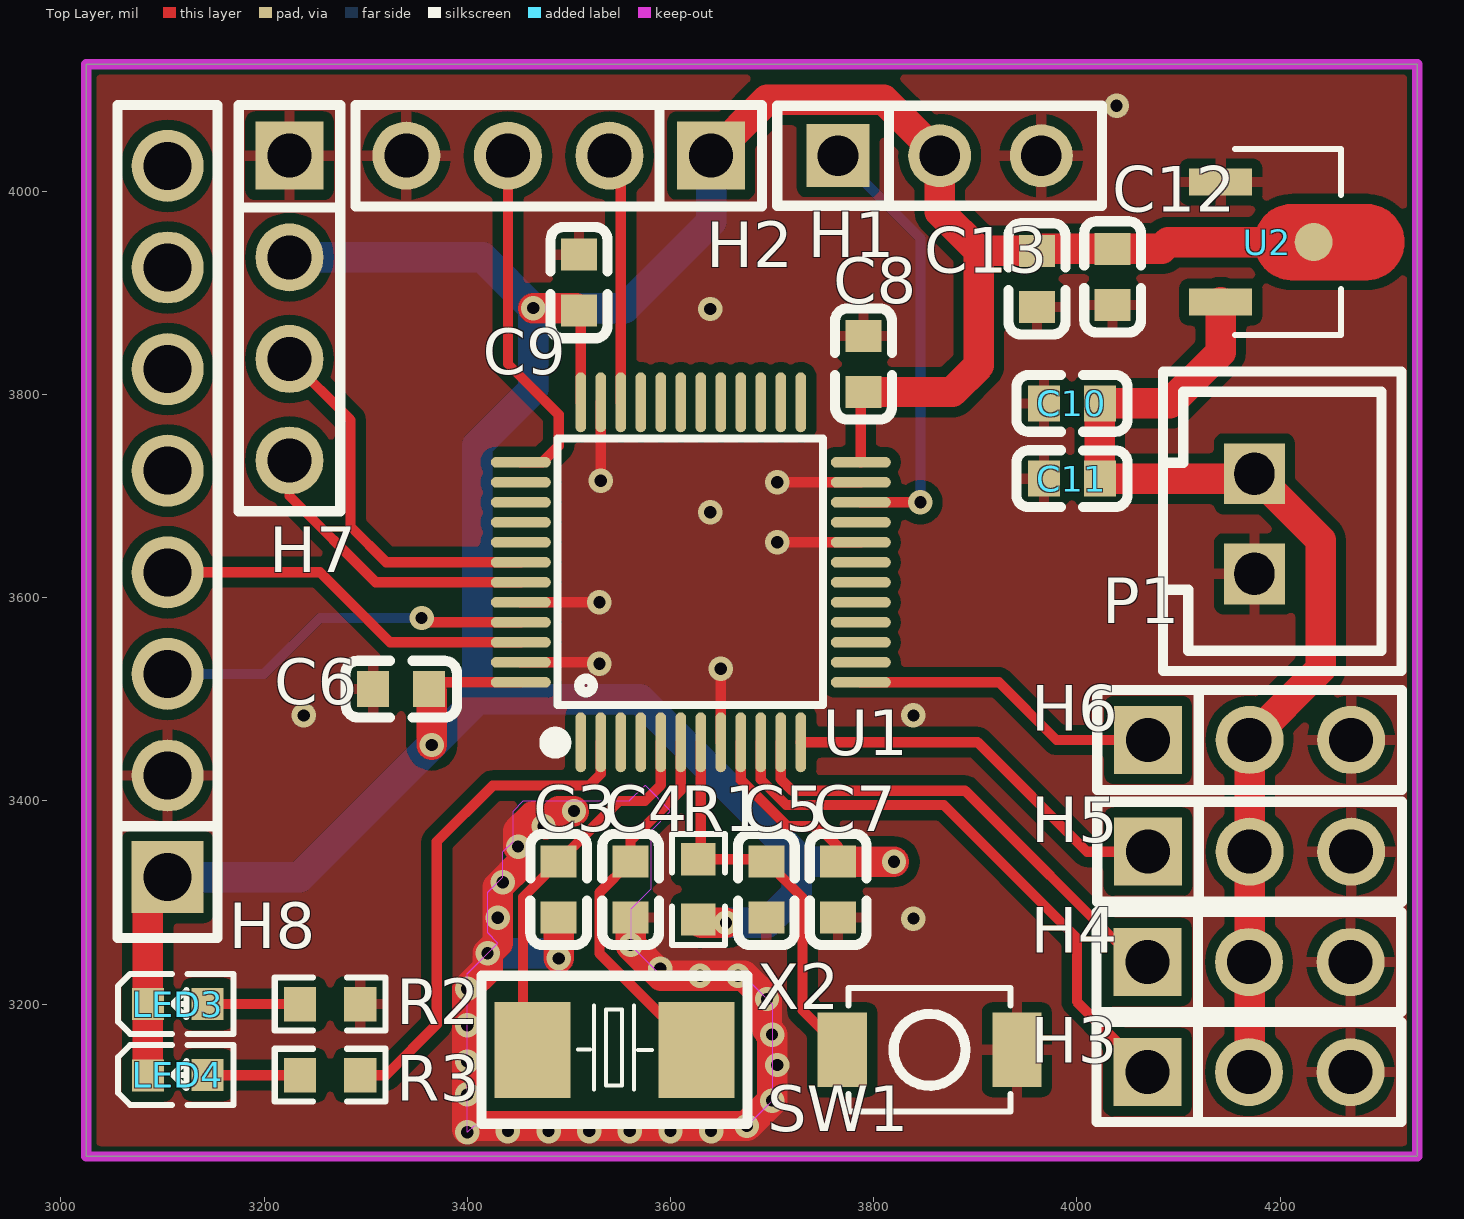
[diagram p0: Top Layer view]
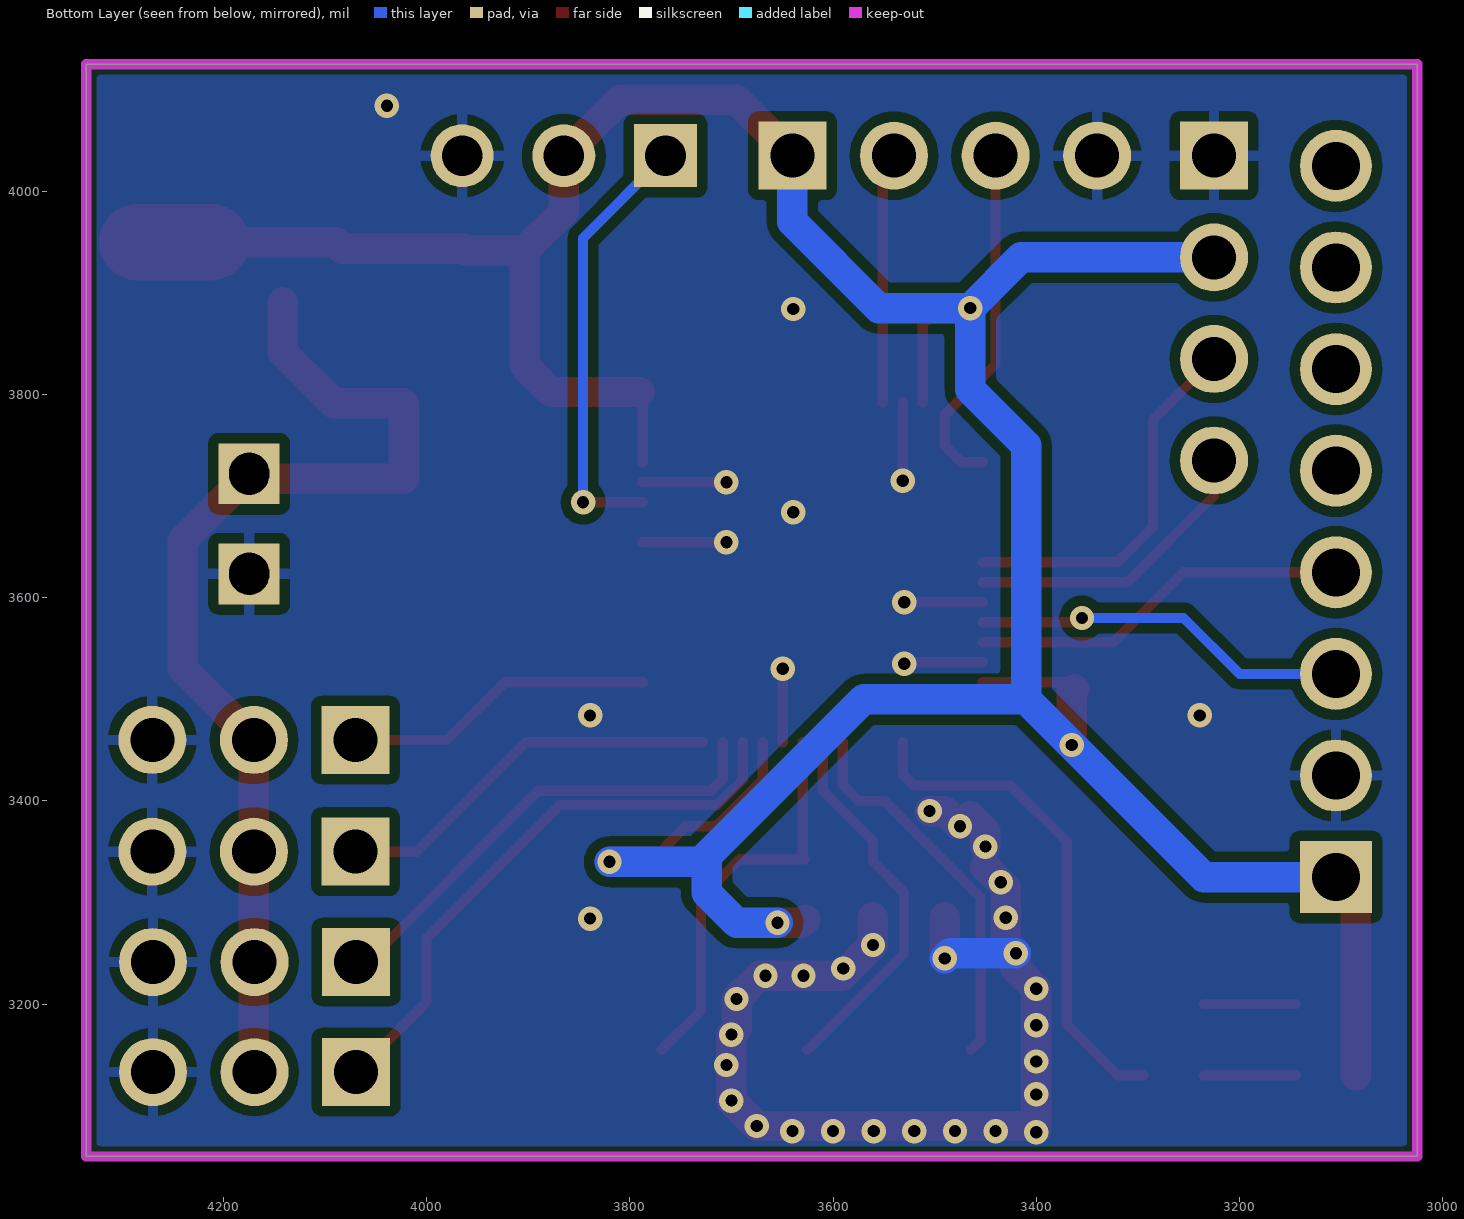
[diagram p1: Bottom Layer view, seen from below]
# Altium PCB MISC51388.pcbdoc
Units mil, origin at the board's own origin, x right, y up, seen from the top; angles counter-clockwise.
Board outline 1310 x 1075 mil, 2 copper layers (Top Layer, Bottom Layer), stack 62.206 mil thick; 29 components, 22 nets, 120 pads, 45 vias.

## Layer stack, top to bottom
Top Solder Mask Layer: solder mask 0.394, Dk 3.3
Top Layer: signal copper 1.379
Dielectric1: surface 59.449, FR4, Dk 4.5
Bottom Layer: signal copper 1.378
Bottom Solder Mask Layer: solder mask 0.394, Dk 3.3

## Board outline
3025,4125 3025,3050 4335,3050 4335,4125

## Design rules (kind name [scope] priority, off if disabled: settings)
BoardOutlineClearance copperThickness2oz_1 [All] p2 off: genericclearance=7.99 ignorepadtopadclearanceinfootprint=FALSE except(0: Arc-SplitContinuation Track-SplitContinuation SMDPad-SplitContinuation THPad-SplitContinuation Via-SplitContinuation Fill-SplitContinuation Region-SplitContinuation Poly-SplitContinuation Text-SplitContinuation Hole-SplitContinuation; 5.98: Arc-CutoutEdge Track-CutoutEdge SMDPad-CutoutEdge THPad-CutoutEdge Via-CutoutEdge Text-CutoutEdge; 6.9: Hole-OutlineEdge Hole-CutoutEdge; 10: Poly-OutlineEdge Poly-CutoutEdge; 11.81: Arc-OutlineEdge Track-OutlineEdge SMDPad-OutlineEdge THPad-OutlineEdge Via-OutlineEdge Fill-OutlineEdge Region-OutlineEdge Text-OutlineEdge Fill-CutoutEdge Region-CutoutEdge)
BoardOutlineClearance Plane_innerPlane_1 [All] p4 off: genericclearance=4.02 ignorepadtopadclearanceinfootprint=FALSE except(0: Arc-SplitContinuation Track-SplitContinuation SMDPad-SplitContinuation THPad-SplitContinuation Via-SplitContinuation Fill-SplitContinuation Region-SplitContinuation Poly-SplitContinuation Text-SplitContinuation Hole-SplitContinuation; 5.98: SMDPad-CutoutEdge THPad-CutoutEdge Via-CutoutEdge Fill-CutoutEdge Region-CutoutEdge Text-CutoutEdge; 6.93: Hole-OutlineEdge Hole-CutoutEdge; 10: Poly-OutlineEdge Poly-CutoutEdge; 11.81: Arc-OutlineEdge Track-OutlineEdge SMDPad-OutlineEdge THPad-OutlineEdge Via-OutlineEdge Fill-OutlineEdge Region-OutlineEdge Text-OutlineEdge Arc-CutoutEdge Track-CutoutEdge)
BoardOutlineClearance Copper_copperRegion_1 [All] p6 off: genericclearance=4.02 ignorepadtopadclearanceinfootprint=FALSE except(0: Arc-SplitContinuation Track-SplitContinuation SMDPad-SplitContinuation THPad-SplitContinuation Via-SplitContinuation Fill-SplitContinuation Region-SplitContinuation Poly-SplitContinuation Text-SplitContinuation Hole-SplitContinuation; 5.98: SMDPad-CutoutEdge THPad-CutoutEdge Via-CutoutEdge Fill-CutoutEdge Region-CutoutEdge Text-CutoutEdge; 6.93: Hole-OutlineEdge Hole-CutoutEdge; 10: Poly-OutlineEdge Poly-CutoutEdge; 11.81: Arc-OutlineEdge Track-OutlineEdge SMDPad-OutlineEdge THPad-OutlineEdge Via-OutlineEdge Fill-OutlineEdge Region-OutlineEdge Text-OutlineEdge Arc-CutoutEdge Track-CutoutEdge)
BoardOutlineClearance copperThickness1oz_1 [All] p8: genericclearance=4.02 ignorepadtopadclearanceinfootprint=FALSE except(0: Arc-SplitContinuation Track-SplitContinuation SMDPad-SplitContinuation THPad-SplitContinuation Via-SplitContinuation Fill-SplitContinuation Region-SplitContinuation Poly-SplitContinuation Text-SplitContinuation Hole-SplitContinuation; 5.98: SMDPad-CutoutEdge THPad-CutoutEdge Via-CutoutEdge Fill-CutoutEdge Region-CutoutEdge Text-CutoutEdge; 6.93: Hole-OutlineEdge Hole-CutoutEdge; 10: Poly-OutlineEdge Poly-CutoutEdge; 11.81: Arc-OutlineEdge Track-OutlineEdge SMDPad-OutlineEdge THPad-OutlineEdge Via-OutlineEdge Fill-OutlineEdge Region-OutlineEdge Text-OutlineEdge Arc-CutoutEdge Track-CutoutEdge)
Clearance copperThickness2oz [All] p1 off: gap=7.99 ignorepadtopadclearanceinfootprint=FALSE except(5.98: SMDPad-Track SMDPad-SMDPad THPad-Track SMDPad-THPad THPad-THPad Track-Via SMDPad-Via THPad-Via Via-Via Fill-SMDPad Region-SMDPad Fill-THPad Region-THPad Fill-Via Region-Via Fill-Fill Fill-Region Region-Region Arc-Track Arc-SMDPad Arc-THPad Arc-Via Fill-Arc Region-Arc Arc-Arc Text-Track SMDPad-Text Text-THPad Text-Via Fill-Text Region-Text Arc-Text Text-Text; 6.9: Hole-Track Hole-SMDPad Hole-THPad Hole-Via Fill-Hole Region-Hole Hole-Arc Hole-Text; 10: Poly-Track Poly-SMDPad Poly-THPad Poly-Via Poly-Fill Poly-Region Poly-Poly Poly-Arc Poly-Text Poly-Hole; 11.81: Fill-Track Region-Track)
Clearance Plane_innerPlane [All] p3 off: gap=4.02 ignorepadtopadclearanceinfootprint=FALSE except(5.98: SMDPad-Track SMDPad-SMDPad THPad-Track SMDPad-THPad THPad-THPad Track-Via SMDPad-Via THPad-Via Via-Via Fill-Track Region-Track Fill-SMDPad Region-SMDPad Fill-THPad Region-THPad Fill-Via Region-Via Fill-Fill Fill-Region Region-Region Arc-Track Arc-SMDPad Arc-THPad Arc-Via Fill-Arc Region-Arc Arc-Arc Text-Track SMDPad-Text Text-THPad Text-Via Fill-Text Region-Text Arc-Text Text-Text; 6.93: Hole-Track Hole-SMDPad Hole-THPad Hole-Via Fill-Hole Region-Hole Hole-Arc Hole-Text; 10: Poly-Track Poly-SMDPad Poly-THPad Poly-Via Poly-Fill Poly-Region Poly-Poly Poly-Arc Poly-Text Poly-Hole)
Clearance Copper_copperRegion [All] p5 off: gap=4.02 ignorepadtopadclearanceinfootprint=FALSE except(5.98: SMDPad-Track SMDPad-SMDPad THPad-Track SMDPad-THPad THPad-THPad Track-Via SMDPad-Via THPad-Via Via-Via Fill-Track Region-Track Fill-SMDPad Region-SMDPad Fill-THPad Region-THPad Fill-Via Region-Via Fill-Fill Fill-Region Region-Region Arc-Track Arc-SMDPad Arc-THPad Arc-Via Fill-Arc Region-Arc Arc-Arc Text-Track SMDPad-Text Text-THPad Text-Via Fill-Text Region-Text Arc-Text Text-Text; 6.93: Hole-Track Hole-SMDPad Hole-THPad Hole-Via Fill-Hole Region-Hole Hole-Arc Hole-Text; 10: Poly-Track Poly-SMDPad Poly-THPad Poly-Via Poly-Fill Poly-Region Poly-Poly Poly-Arc Poly-Text Poly-Hole)
Clearance copperThickness1oz [All] p7: gap=4.02 ignorepadtopadclearanceinfootprint=FALSE except(5.98: SMDPad-Track SMDPad-SMDPad THPad-Track SMDPad-THPad THPad-THPad Track-Via SMDPad-Via THPad-Via Via-Via Fill-Track Region-Track Fill-SMDPad Region-SMDPad Fill-THPad Region-THPad Fill-Via Region-Via Fill-Fill Fill-Region Region-Region Arc-Track Arc-SMDPad Arc-THPad Arc-Via Fill-Arc Region-Arc Arc-Arc Text-Track SMDPad-Text Text-THPad Text-Via Fill-Text Region-Text Arc-Text Text-Text; 6.93: Hole-Track Hole-SMDPad Hole-THPad Hole-Via Fill-Hole Region-Hole Hole-Arc Hole-Text; 10: Poly-Track Poly-SMDPad Poly-THPad Poly-Via Poly-Fill Poly-Region Poly-Poly Poly-Arc Poly-Text Poly-Hole)
DiffPairsRouting differentialPair [All] p1: maxlimit=6 minlimit=6 mostfreqgap=6 toplayer_minwidth=5 toplayer_prefwidth=10 toplayer_maxwidth=100 toplayer_mingap=6 toplayer_prefgap=6 toplayer_maxgap=6 bottomlayer_minwidth=5 bottomlayer_prefwidth=10 bottomlayer_maxwidth=100 bottomlayer_mingap=6 bottomlayer_prefgap=6 bottomlayer_maxgap=6 maxuncoupledlength=10
HoleToHoleClearance otherClearance [All] p1: gap=11.81 allowstackedmicrovias=TRUE
Length netLength [All] p1: minlimit=0 maxlimit=0
PasteMaskExpansion pasteMaskExpansion [All] p1: expansion=0
PlaneConnect innerPlane [All] p1: planeconnectstyle=Relief reliefexpansion=20 reliefentries=4 reliefconductorwidth=10 reliefairgap=10
PolygonConnect copperRegion [All] p1: connectstyle=Relief reliefconductorwidth=10 reliefentries=4 polygonreliefangle="90 Angle" airgapwidth=10 via.connectstyle=Relief via.reliefconductorwidth=10 via.reliefentries=4 via.polygonreliefangle="90 Angle" via.airgapwidth=10
RoutingVias viaSize [All] p1: holewidth=12.01 width=24.02 viastyle="Through Hole" minholewidth=11.81 minwidth=19.68 maxholewidth=248.03 maxwidth=393.7
SolderMaskExpansion solderMaskExpansion [IsVia] p1: expansion=-1000 istentingtop=TRUE
SolderMaskExpansion solderMaskExpansion [All] p2: expansion=2 istentingtop=FALSE
Width copperThickness2oz_2 [All] p1 off: maxlimit=100 minlimit=8 preferedwidth=10
Width copperThickness1oz_2 [All] p2: maxlimit=100 minlimit=5 preferedwidth=20

## Components (designator, comment, footprint, x,y, rotation, side; value= is the part's Value field where it differs from the comment)
C3 "20pF" C0603 3490,3312.85 r90 top
C4 "20pF" C0603 3560.72,3312.85 r90 top
C5 "100nF" C0603 3694.28,3312.85 r90 top
C6 "100nF" C0603 3335,3510 r0 top
C7 "100nF" C0603 3765,3312.85 r90 top
C8 "100nF" C0603 3790,3830 r270 top
C9 "100nF" C0603 3510,3910 r270 top
C10 "100nF" C0603 3995.12,3791.22 r0 top
C11 "10uF" C0603 3995.12,3717.09 r0 top
C12 "100nF" C0603 4035.14,3915.79 r90 top
C13 "10uF" C0603 3960.76,3913.83 r90 top
H1 "" HDR-TH_3P-P2.54-V-F 3865,4035 r0 top
H2 "PZ254V-11-04P" HDR-TH_4P-P2.54-V-M 3490,4035 r180 top
H3 "" HDR-TH_3P-P2.54-V-M 4169.37,3133.05 r0 top
H4 "" HDR-TH_3P-P2.54-V-M 4169.37,3241.38 r0 top
H5 "" HDR-TH_3P-P2.54-V-M 4170,3350 r0 top
H6 "" HDR-TH_3P-P2.54-V-M 4170,3460 r0 top
H7 "PZ254V-11-04P" HDR-TH_4P-P2.54-V-M 3225,3885 r270 top
H8 "" HDR-TH_8P-P2.54-V-F-1 3105,3675 r90 top
LED3 "LTST-C190YKT" LED0603-RD 3115,3200 r0 top
LED4 "GL0603UB01" LED0603-RD_BLUE 3115,3130 r0 top
P1 "XH2.54直插座-2P" CONN-TH_XH2.54-2P 4174.67,3672.75 r270 top
R1 "10kΩ" R0603 3627.5,3312.85 r270 top
R2 "680Ω" R0603 3265,3200 r0 top
R3 "680Ω" R0603 3265,3130 r0 top
SW1 "TS-1088-AR02016" SW-SMD_L3.9-W3.0-P4.45 3855,3155 r0 top
U1 "STM32F103C8T6" LQFP-48_L7.0-W7.0-P0.50-LS9.0-BL 3620,3625 r0 top
U2 "AMS1117-1.2OFB" SOT-89-3_L4.5-W2.4-P1.50-LS4.0-BR 4195,3950 r180 top
X2 "8MHz" CRYSTAL-SMD_L5.0-W3.2 3545,3155 r180 top

## Footprints (in the part's own frame and the unit in brackets; to place one, negate y for a bottom-side part, rotate by r counter-clockwise, add the part's x,y. Pads: shape width x height; smd on the part's side, far side on the other; paste and mask are expansions set on the pad)
C0603 [mm]
  rect 0.8x0.9 smd: 1(-0.7,0) 2(0.7,0)
  silkscreen extent -1.39,-0.71 1.39,0.71
CONN-TH_XH2.54-2P [mil]
  rect 60x60 hole 39.37 slot 41.34 at 0 deg paste+0 mask+1.97: 1(-49.22,0) 2(49.21,0)
  silkscreen extent -150,-90 145,145
CRYSTAL-SMD_L5.0-W3.2 [mm]
  rect 1.9x2.4 smd: 1(-2.05,0) 2(2.05,0)
  silkscreen extent -3.32,-1.85 3.33,1.85
HDR-TH_3P-P2.54-V-F [mil]
  rect 62x62 hole 40.16: 1(-100,0)
  round 62 hole 40.16: 2(0,0) 3(100,0)
  silkscreen extent -160,-49 160,49
HDR-TH_3P-P2.54-V-M [mm]
  rect 1.7x1.7 hole 1.1: 1(-2.54,0)
  round 1.7 hole 1.1: 2(0,0) 3(2.54,0)
  silkscreen extent -3.81,-1.25 3.81,1.25
HDR-TH_4P-P2.54-V-M [mm]
  rect 1.7x1.7 hole 1.1: 1(-3.81,0)
  round 1.7 hole 1.1: 2(-1.27,0) 3(1.27,0) 4(3.81,0)
  silkscreen extent -5.08,-1.27 5.08,1.27
HDR-TH_8P-P2.54-V-F-1 [mm]
  rect 1.8x1.8 hole 1.2: 1(-8.89,0)
  round 1.8 hole 1.2: 2(-6.35,0) 3(-3.81,0) 4(-1.27,0) 5(1.27,0) 6(3.81,0) 7(6.35,0) 8(8.89,0)
  silkscreen extent -10.41,-1.25 10.41,1.25
LED0603-RD [mm]
  rect 0.8x0.8 smd: 1(-0.749,0) 2(0.749,0)
  silkscreen extent -1.49,-0.75 1.39,0.76
LED0603-RD_BLUE [mm]
  rect 0.8x0.8 smd: 1(-0.749,-0.004) 2(0.749,0.004)
  silkscreen extent -1.49,-0.75 1.39,0.76
LQFP-48_L7.0-W7.0-P0.50-LS9.0-BL [mm]
  oval 0.27x1.5 smd paste+0 mask+0.05: 1(-2.75,-4.25) 2(-2.25,-4.25) 3(-1.75,-4.25) 4(-1.25,-4.25) 5(-0.75,-4.25) 6(-0.25,-4.25) 7(0.25,-4.25) 8(0.75,-4.25) 9(1.25,-4.25) 10(1.75,-4.25) 11(2.25,-4.25) 12(2.75,-4.25) 25(2.75,4.25) 26(2.25,4.25) 27(1.75,4.25) 28(1.25,4.25) 29(0.75,4.25) 30(0.25,4.25) 31(-0.25,4.25) 32(-0.75,4.25) 33(-1.25,4.25) 34(-1.75,4.25) 35(-2.25,4.25) 36(-2.75,4.25)
  oval 1.5x0.27 smd paste+0 mask+0.05: 13(4.25,-2.75) 14(4.25,-2.25) 15(4.25,-1.75) 16(4.25,-1.25) 17(4.25,-0.75) 18(4.25,-0.25) 19(4.25,0.25) 20(4.25,0.75) 21(4.25,1.25) 22(4.25,1.75) 23(4.25,2.25) 24(4.25,2.75) 37(-4.25,2.75) 38(-4.25,2.25) 39(-4.25,1.75) 40(-4.25,1.25) 41(-4.25,0.75) 42(-4.25,0.25) 43(-4.25,-0.25) 44(-4.25,-0.75) 45(-4.25,-1.25) 46(-4.25,-1.75) 47(-4.25,-2.25) 48(-4.25,-2.75)
  silkscreen extent -3.59,-4.46 3.3,3.34
R0603 [mil]
  rect 31.75x34.02 smd paste-3937.01 mask+2: 1(-29.66,0) 2(29.66,0)
  silkscreen extent -55,-26 55,26
SOT-89-3_L4.5-W2.4-P1.50-LS4.0-BR [mm]
  rect 1.575x0.672 smd: 1(1.356,-1.5) 3(1.356,1.5)
  round 0.95 smd: 2(-0.966,0)
  Top Layer region: -2.283,0.95 -0.429,0.95 -0.384,0.949 -0.34,0.946 -0.296,0.941 -0.252,0.933 -0.208,0.924 -0.165,0.913 -0.123,0.899 -0.081,0.884 -0.04,0.867 0,0.847 0.04,0.826 0.078,0.804 0.115,0.779 0.151,0.753 0.185,0.725 0.219,0.695 0.251,0.664 0.281,0.631 0.31,0.597 0.337,0.562 0.362,0.525 0.386,0.488 0.408,0.449 0.428,0.409 0.447,0.33 2.144,0.33 2.144,-0.33 0.447,-0.33 0.428,-0.409 0.408,-0.449 0.386,-0.488 0.362,-0.525 0.337,-0.562 0.31,-0.597 0.281,-0.631 0.251,-0.664 0.219,-0.695 0.185,-0.725 0.151,-0.753 0.115,-0.779 0.078,-0.804 0.04,-0.826 0,-0.847 -0.04,-0.867 -0.081,-0.884 -0.123,-0.899 -0.165,-0.913 -0.208,-0.924 -0.252,-0.933 -0.296,-0.941 -0.34,-0.946 -0.384,-0.949 -0.429,-0.95 -2.283,-0.95 -2.328,-0.949 -2.372,-0.946 -2.416,-0.941 -2.46,-0.933 -2.504,-0.924 -2.547,-0.913 -2.589,-0.899 -2.631,-0.884 -2.672,-0.867 -2.712,-0.847 -2.752,-0.826 -2.79,-0.804 -2.827,-0.779 -2.863,-0.753 -2.898,-0.725 -2.931,-0.695 -2.963,-0.664 -2.993,-0.631 -3.022,-0.597 -3.049,-0.562 -3.075,-0.525 -3.098,-0.488 -3.12,-0.449 -3.14,-0.409 -3.159,-0.369 -3.175,-0.327 -3.189,-0.285 -3.202,-0.242 -3.212,-0.199 -3.22,-0.155 -3.227,-0.111 -3.231,-0.067 -3.233,-0.022 -3.233,0.022 -3.231,0.067 -3.227,0.111 -3.22,0.155 -3.212,0.199 -3.202,0.242 -3.189,0.285 -3.175,0.327 -3.159,0.369 -3.14,0.409 -3.12,0.449 -3.098,0.488 -3.075,0.525 -3.049,0.562 -3.022,0.597 -2.993,0.631 -2.963,0.664 -2.931,0.695 -2.898,0.725 -2.863,0.753 -2.827,0.779 -2.79,0.804 -2.752,0.826 -2.712,0.847 -2.672,0.867 -2.631,0.884 -2.589,0.899 -2.547,0.913 -2.504,0.924 -2.46,0.933 -2.416,0.941 -2.372,0.946 -2.328,0.949
  silkscreen extent -1.65,-2.33 1,2.33
SW-SMD_L3.9-W3.0-P4.45 [mm]
  rect 1.23x1.86 smd: 1(-2.185,0) 2(2.185,0)
  silkscreen extent -2.03,-1.54 2.03,1.54

## Via types
v1: diameter 24.02, hole 12, Top Layer to Bottom Layer, 45 vias

## Nets (pads, with @x,y where several pads share a name; then routed paths per layer and width w, separated by ;. In a path a pad name is that pad's centre, name@x,y a point inside that pad or via, vN(x,y) a via of type N, cw(c..) or ccw(c..) an arc to the next point about the centre after c; other vN are vias at no path point)
$1N1710: LED3.2 R2.1 | length 90.8
  Top Layer w10: LED3.2 R2.1
$1N1749: LED4.2 R3.1 | length 90.9
  Top Layer w10: LED4.2 3144.63,3130 R3.1
+5V: C10.2 C11.2 H3.2 H4.2 H5.2 H6.2 P1.1 U2.3 | length 1062.5
  Top Layer w30: U2.3 4141.6,3841.6 4091.22,3791.22 C10.2 C11.2 4169.8,3717.09 P1.1 4240,3656.64 4240,3530 H6.2 H5.2 4170,3133.68 H3.2
GND: C3.1 C4.1 C5.1 C6.1 C7.1 C8.1 C9.1 C10.1 C11.1 C12.1 C13.1 H1.3 H2.4 H3.3 H4.3 H5.3 H6.3 H7.1 H8.2 P1.2 R2.2 SW1.2 U1.8 U1.20 U1.23 U1.35 U1.44 U1.47 U2.1 | length 1519.9
  Top Layer w10: U1.47 3528.58,3536.42 v1(3530,3535) ; U1.44 v1(3530,3595.47) ; v1(3531.42,3715) U1.35 ; U1.8 v1(3649.53,3530) ; v1(3705,3654.53) U1.20 ; v1(3705,3713.58) U1.23
  Top Layer w30: v1@3400,3076.81 v1(3400,3111.12) v1(3400,3143.51) v1(3400,3179.24) v1(3400,3215) 3420,3235 v1(3420,3250) 3430,3260 v1(3430,3285) 3430,3315 v1(3435,3320) 3450,3335 ; v1@3406.18,3080 v1(3675,3080) v1(3700,3105) v1(3700,3170) 3695,3175 v1(3695,3205) 3672.16,3227.84 v1(3629.05,3227.84) 3591,3227.84 v1(3560.71,3258.13) C4.1 ; v1(3450,3355) 3450,3370 3465,3385 ; v1@3477.14,3377.14 3490,3390 v1(3505,3390) ; v1(3490,3245) C3.1
  Bottom Layer w30: v1(3420,3250) 3485,3250 v1(3490,3245)
  other v1: 3400,3073.82 3440,3075 3480,3075 3520,3075 3560,3075 3600,3075 3640,3075 3705,3140 3666.46,3227.84 3590,3235 3839.1,3284.1 3475,3375 3239.1,3484.1 3839.1,3484.1 3639.1,3684.1 3639.1,3884.1 4039.1,4084.1
NRST: C5.2 R1.1 SW1.1 U1.7 | length 400.1
  Top Layer w10: U1.7 3629.84,3344.85 R1.1 3692.17,3342.51 C5.2 3730,3304.68 3730,3193.98 SW1.1
OSCIN: C3.2 U1.5 X2.2 | length 377.5
  Top Layer w10: X2.2 3455,3164.29 3455,3305.41 C3.2 3549.59,3400 3575,3400 3590.47,3415.47 U1.5
OSCOUT: C4.2 U1.6 X2.1 | length 375.9
  Top Layer w10: U1.6 3610.16,3410.16 3560.72,3360.72 C4.2 3530,3309.68 3530,3250 3625,3155 X2.1
OUT: H1.1 U1.22 | length 433.3
  Top Layer w10: U1.22 v1(3845.99,3693.9)
  Bottom Layer w10: H1.1 3845.99,3954.01 v1(3845.99,3693.9)
PA0: H3.1 U1.10 | length 573
  Top Layer w10: U1.10 3688.9,3421.1 3714.02,3395.98 3869.02,3395.98 4000,3265 4000,3202.42 H3.1
PA1: H4.1 U1.11 | length 471.6
  Top Layer w10: U1.11 3708.58,3421.42 3720,3410 3890,3410 4058.62,3241.38 H4.1
PA2: H5.1 U1.12 | length 386.3
  Top Layer w10: U1.12 3902.32,3457.68 4010,3350 H5.1
PA3: H6.1 U1.13 | length 306.2
  Top Layer w10: U1.13 3923.27,3516.73 3980,3460 H6.1
PB8: H8.3 U1.45 | length 372.2
  Top Layer w10: v1(3355,3580) 3359.21,3575.79 U1.45
  Bottom Layer w10: H8.3 3200,3525 3255,3580 v1(3355,3580)
PB9: H8.4 U1.46 | length 376.2
  Top Layer w10: H8.4 3255,3625 3323.9,3556.1 U1.46
PC13: R3.2 U1.2 | length 496.2
  Top Layer w10: R3.2 3320,3130 3370,3180 3370,3360 3425,3415 3520,3415 3531.42,3426.42 U1.2
PC14: U1.3
PC15: U1.4
SCL: H7.3 U1.42 | length 372.1
  Top Layer w10: H7.3 3285,3775 3285,3670 3320.16,3634.84 U1.42
SDA: H7.4 U1.43 | length 297.8
  Top Layer w10: H7.4 3225,3700 3309.84,3615.16 U1.43
SWCLK: H2.3 U1.37 | length 350.3
  Top Layer w10: H2.3 3440,3830 3490,3780 3490,3749.4 3473.87,3733.27 U1.37
SWIO: H2.2 U1.34 | length 247.3
  Top Layer w10: H2.2 3551.1,4023.9 U1.34
VCC3V3: C6.2 C7.2 C8.2 C9.2 C12.2 C13.2 H1.2 H2.1 H7.2 H8.1 LED3.1 LED4.1 R1.2 U1.9 U1.24 U1.36 U1.48 U2.2 | length 3694
  Top Layer w10: C6.2 3369.29,3516.73 U1.48 ; U1.36 C9.2@3511.73,3880.71 ; U1.9 3669.21,3420.79 3715,3375 3745,3375 3765,3355 C7.2 ; U1.24 3787.32,3799.76 C8.2
  Top Layer w30: LED4.1 LED3.1 3085.51,3305.51 H8.1 ; C6.2 3365,3507.56 v1(3365,3455) ; v1(3465,3885) 3507.44,3885 C9.2 ; R1.2 3630.69,3280 v1(3654.64,3280) ; H2.1 3695,4090 3810,4090 H1.2 3865,3980 3903.61,3941.39 ; C7.2 3765.41,3340 v1(3820,3340) ; C8.2 3877.44,3802.44 3903.61,3828.61 3903.61,3941.39 ; U2.2@4248.4,3950.01 4090.01,3950.01 4083.35,3943.35 C12.2 3962.72,3943.35 C13.2 3903.61,3941.39
  Bottom Layer w30: H8.1 3235,3325 v1(3365,3455) 3410,3500 ; H7.2 3415,3935 v1(3465,3885) ; H2.1 3640,3970 3555,3885 v1(3465,3885) ; v1(3654.64,3280) 3695,3280 3724.51,3309.51 3724.51,3340 ; v1(3820,3340) 3724.51,3340 ; 3410,3500 3410,3750 3465,3805 v1(3465,3885) ; 3410,3500 3570,3500 3724.51,3345.49 3724.51,3340
pads on no net: H8.5 H8.6 H8.7 H8.8 U1.1 U1.14 U1.15 U1.16 U1.17 U1.18 U1.19 U1.21 U1.25 U1.26 U1.27 U1.28 U1.29 U1.30 U1.31 U1.32 U1.33 U1.38 U1.39 U1.40 U1.41

## Polygon pours and split planes (outlines as drawn)
GND on Top Layer (solid, remove dead copper, pour order 2): 3000,4160 3000,3000 4669.9,3000 4669.9,4160
GND on Bottom Layer (solid, remove dead copper, pour order 2): 3000,4160 3000,3010 4675,3010 4675,4160

## Keep-outs
Top Layer:
  region: 3575,3415.47 3600,3390.47 3600,3390 3580.34,3370.34 3580.34,3312.85 3560.71,3293.22 3560.71,3258.13 3591,3227.84 3672.16,3227.84 3700,3200 3700,3105 3675,3080 3406.18,3080 3400,3073.82 3400,3230 3430,3260 3420,3270 3420,3310 3435,3325 3435,3350 3445,3360 3445,3390 3455,3400 3559.53,3400
Board Outline Layer:
  the board outline again, w10